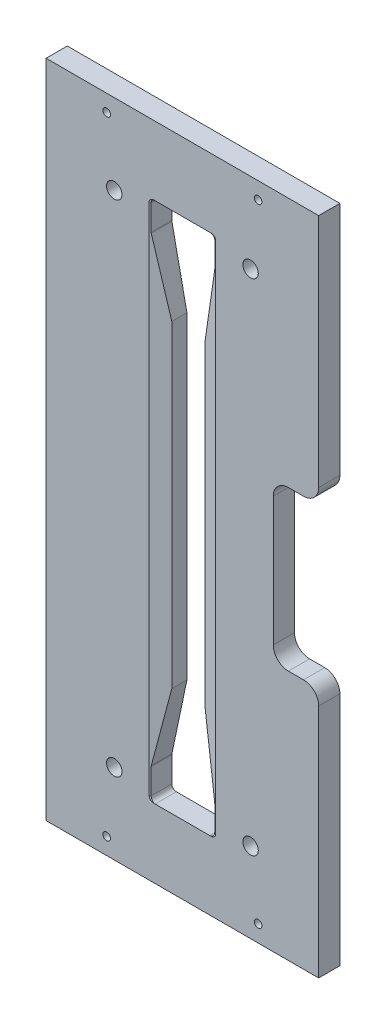
from build123d import *

# Parameters (mm, degrees)
SKETCH1_W              = 180
SKETCH1_H              = 436
BOSS_EXTRUDE1_DEPTH    = 14
SKETCH5_W              = 30
SKETCH5_H              = 105
CUT_EXTRUDE1_DEPTH     = 472.902532309
M12_TAPPED_HOLE1_D     = 10.2
M12_TAPPED_HOLE1_DEPTH = 32.75
M12_TAPPED_HOLE1_TIP   = 3.064389157
FILLET1_R              = 10
M6_TAPPED_HOLE1_D      = 5
M6_TAPPED_HOLE1_DEPTH  = 17
M6_TAPPED_HOLE1_TIP    = 1.502151548
CUT_EXTRUDE2_DEPTH     = 5
CUT_EXTRUDE2_DRAFT     = -70


with BuildPart() as part:
    # Sketch1 → Boss-Extrude1 (new body)
    with BuildSketch(Plane.XY):
        with Locations((90, 218)):
            Rectangle(SKETCH1_W, SKETCH1_H)
        with BuildLine():
            Line((72, 45.5), (108, 45.5))
            ThreePointArc((108, 45.5), (110.121320344, 46.378679656), (111, 48.5))
            Line((111, 48.5), (111, 65.187634121))
            ThreePointArc((111, 65.187634121), (110.98386897, 65.498320406), (110.935649355, 65.805665564))
            Line((110.935649355, 65.805665564), (101, 113))
            Line((101, 113), (101, 323))
            Line((101, 323), (110.935649355, 370.194334436))
            ThreePointArc((110.935649355, 370.194334436), (110.98386897, 370.501679594), (111, 370.812365879))
            Line((111, 370.812365879), (111, 387.5))
            ThreePointArc((111, 387.5), (110.121320344, 389.621320344), (108, 390.5))
            Line((108, 390.5), (72, 390.5))
            ThreePointArc((72, 390.5), (69.878679656, 389.621320344), (69, 387.5))
            Line((69, 387.5), (69, 370.812365879))
            ThreePointArc((69, 370.812365879), (69.01613103, 370.501679594), (69.064350645, 370.194334436))
            Line((69.064350645, 370.194334436), (79, 323))
            Line((79, 323), (79, 113))
            Line((79, 113), (69.064350645, 65.805665564))
            ThreePointArc((69.064350645, 65.805665564), (69.01613103, 65.498320406), (69, 65.187634121))
            Line((69, 65.187634121), (69, 48.5))
            ThreePointArc((69, 48.5), (69.878679656, 46.378679656), (72, 45.5))
        make_face(mode=Mode.SUBTRACT)
    extrude(amount=-BOSS_EXTRUDE1_DEPTH)

    # Sketch5 → Cut-Extrude1 (cut, through all)
    with BuildSketch(Plane.XY):
        with Locations((165, 218)):
            Rectangle(SKETCH5_W, SKETCH5_H)
    extrude(amount=-CUT_EXTRUDE1_DEPTH, mode=Mode.SUBTRACT)

    # M12 Tapped Hole1
    with Locations(Plane(origin=(0, 0, -14), x_dir=(-1, 0, 0), z_dir=(0, 0, -1))):
        with Locations((-135, 383), (-45, 383), (-45, 53), (-135, 53)):
            Hole(M12_TAPPED_HOLE1_D / 2, depth=M12_TAPPED_HOLE1_DEPTH)
            with Locations((0, 0, -(M12_TAPPED_HOLE1_DEPTH + M12_TAPPED_HOLE1_TIP / 2))):  # 118° drill point
                Cone(0, M12_TAPPED_HOLE1_D / 2, M12_TAPPED_HOLE1_TIP, mode=Mode.SUBTRACT)

    # Fillet1
    fillet1_edges = [part.edges().sort_by_distance(p)[0] for p in [
        (150, 165.5, -7),
        (150, 270.5, -7),
        (180, 270.5, -7),
        (180, 165.5, -7),
    ]]
    fillet(fillet1_edges, radius=FILLET1_R)

    # M6 Tapped Hole1
    with Locations(Plane.XY):
        with Locations((40, 425), (140, 425), (40, 11), (140, 11)):
            Hole(M6_TAPPED_HOLE1_D / 2, depth=M6_TAPPED_HOLE1_DEPTH)
            with Locations((0, 0, -(M6_TAPPED_HOLE1_DEPTH + M6_TAPPED_HOLE1_TIP / 2))):  # 118° drill point
                Cone(0, M6_TAPPED_HOLE1_D / 2, M6_TAPPED_HOLE1_TIP, mode=Mode.SUBTRACT)


with BuildPart() as cut_extrude2_tool:
    # Sketch8 → Cut-Extrude2 (with draft: the straight prism first)
    with BuildSketch(Plane.XY):
        with BuildLine():
            ThreePointArc((71, 390.5), (68.878679656, 389.621320344), (68, 387.5))
            Line((68, 387.5), (68, 48.5))
            ThreePointArc((68, 48.5), (68.878679656, 46.378679656), (71, 45.5))
            Line((71, 45.5), (109, 45.5))
            ThreePointArc((109, 45.5), (111.121320344, 46.378679656), (112, 48.5))
            Line((112, 48.5), (112, 387.5))
            ThreePointArc((112, 387.5), (111.121320344, 389.621320344), (109, 390.5))
            Line((109, 390.5), (71, 390.5))
        make_face()
    extrude(amount=-CUT_EXTRUDE2_DEPTH)
    # Cut-Extrude2: the draft: its side faces are tilted about the plane it starts from
    cut_extrude2_sides = [cut_extrude2_tool.faces().sort_by_distance(p)[0] for p in [
        (111.121320344, 389.621320344, -2.5),
        (90, 390.5, -2.5),
        (68.878679656, 389.621320344, -2.5),
        (68, 218, -2.5),
        (68.878679656, 46.378679656, -2.5),
        (90, 45.5, -2.5),
        (111.121320344, 46.378679656, -2.5),
        (112, 218, -2.5),
    ]]
    draft(cut_extrude2_sides, Plane.XY, CUT_EXTRUDE2_DRAFT)


with BuildPart() as part_1:
    add(part.part)

    # Cut-Extrude2: cut by cut_extrude2_tool
    add(cut_extrude2_tool.part, mode=Mode.SUBTRACT)


solid = part_1.part
